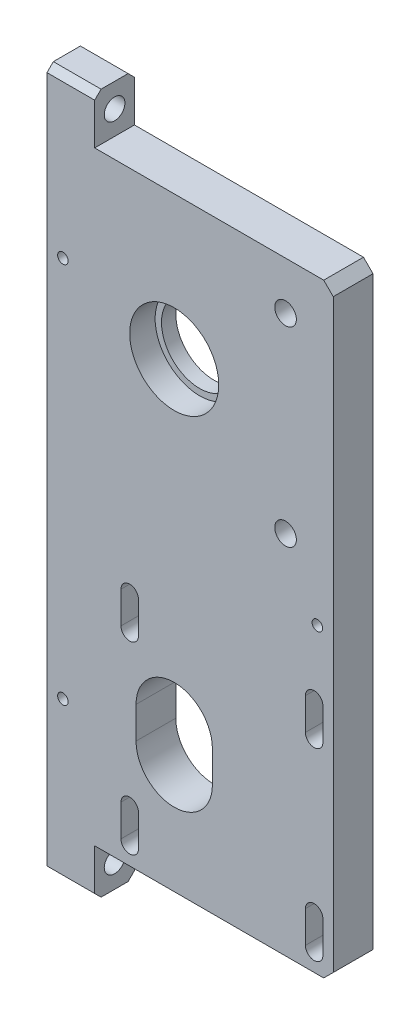
SolidWorks part; units mm, degrees
material "A6061"
ref_plane "前视基准面" through (0, 0, 0) normal (0, 0, 1) x (1, 0, 0)
ref_plane "上视基准面" through (0, 0, 0) normal (0, 1, 0) x (1, 0, 0)
ref_plane "右视基准面" through (0, 0, 0) normal (1, 0, 0) x (0, 0, -1)
sketch "草图1" plane through (0, 0, 0) normal (0, 0, 1) x (1, 0, 0)
  line L0 (0, 0) -> (-90, 0)
  line L1 (-90, 0) -> (-90, 220)
  line L2 (-90, 220) -> (0, 220)
  line L3 (0, 220) -> (0, 0)
  dimension "D1" = 220
  dimension "D4" = 90
extrude "凸台-拉伸1" add sketch "草图1" along normal blind 12.5
sketch "草图2" plane through (0, 0, 12.5) normal (0, 0, 1) x (1, 0, 0)
  line L0 (0, 220) -> (-90, 220) construction
  line L2 (-90, 220) -> (-90, 0) construction
  circle A0 centre (-50, 55) radius 12
  dimension "D1" = 165
  dimension "D2" = 40
  dimension "D3" = 24
extrude "切除-拉伸1" cut sketch "草图2" against normal through all
hole_wizard "打孔尺寸根据内六角圆柱头螺钉的类型1" positions "草图4" profile "草图3" counterbore size "M5" standard "Gb" end condition through all
sketch "草图4" plane through (0, 0, 12.5) normal (0, 0, 1) x (1, 0, 0)
  line L0 (-63.9914, 83.9914) -> (-6.0086, 26.0086) construction
  line L2 (-6.0086, 83.9914) -> (-63.9914, 26.0086) construction
  line L4 (-50, 55) -> (-35, 55) construction
  point P0 (-6.0086, 83.9914)
  point P2 (-6.0086, 26.0086)
  point P4 (-63.9914, 26.0086)
  point P6 (-63.9914, 83.9914)
  dimension "D1" = 45
  dimension "D2" = 90
  dimension "D3" = 15
  dimension "D4" = 82
  dimension "D5" = 82
sketch "草图3" plane through (-6.0086, 83.9914, 12.5) normal (1, 0, 0) x (0, -1, 0)
  line L0 (0, 0) -> (0, 12.5)
  line L1 (0, 12.5) -> (5, 12.5)
  line L3 (5, 12.5) -> (5, 6)
  line L4 (5, 6) -> (2.75, 6)
  line L5 (2.75, 6) -> (2.75, 0)
  line L7 (2.75, 0) -> (0, 0)
  line L11 (0, -6.35) -> (0, 107.95) construction
  dimension "通孔孔直径" = 10
  dimension "通孔孔深度" = 12.5
  dimension "柱形沉头孔直径" = 5.5
  dimension "柱形沉头孔深度" = 6
hole_wizard "M4 螺纹孔1" positions "草图7" profile "草图6" tap size "M4" standard "Gb" end condition through all
sketch "草图7" plane through (0, 0, 12.5) normal (0, 0, 1) x (1, 0, 0)
  line L0 (0, 220) -> (-90, 220) construction
  line L1 (-90, 220) -> (-90, 0) construction
  line L2 (-85, 50) -> (-85, 170) construction
  line L4 (-5, 110) -> (-85, 110) construction
  point P0 (-85, 170)
  point P3 (-85, 50)
  point P13 (-5, 110)
  dimension "D1" = 5
  dimension "D2" = 50
  dimension "D3" = 120
  dimension "D4" = 80
cosmetic thread "孔螺蚊线1" parameters "D2"=4
cosmetic thread "孔螺蚊线2" parameters "D2"=4
sketch "草图6" plane through (-85, 170, 12.5) normal (1, 0, 0) x (0, -1, 0)
  line L0 (0, 0) -> (0, 12.5)
  line L1 (0, 12.5) -> (1.65, 12.5)
  line L2 (1.65, 12.5) -> (1.65, 0)
  line L5 (1.65, 0) -> (0, 0)
  line L11 (0, -6.35) -> (0, 107.95) construction
  dimension "通孔螺纹孔钻头直径" = 3.3
  dimension "通孔螺纹孔钻头深度" = 12.5
cosmetic thread "孔螺蚊线5" parameters "D2"=4
sketch "草图12" plane through (0, 0, 0) normal (0, 0, -1) x (-1, 0, 0)
  line L0 (50, 50) -> (50, 60) construction
  line L1 (38, 50) -> (38, 60)
  line L2 (62, 50) -> (62, 60)
  line L3 (63.9914, 78.9914) -> (63.9914, 88.9914) construction
  line L4 (61.2414, 78.9914) -> (61.2414, 88.9914)
  line L5 (66.7414, 78.9914) -> (66.7414, 88.9914)
  line L6 (63.9914, 31.0086) -> (63.9914, 21.0086) construction
  line L7 (66.7414, 31.0086) -> (66.7414, 21.0086)
  line L8 (61.2414, 31.0086) -> (61.2414, 21.0086)
  line L9 (6.0086, 31.0086) -> (6.0086, 21.0086) construction
  line L10 (8.7586, 31.0086) -> (8.7586, 21.0086)
  line L11 (3.2586, 31.0086) -> (3.2586, 21.0086)
  line L12 (6.0086, 88.9914) -> (6.0086, 78.9914) construction
  line L13 (8.7586, 88.9914) -> (8.7586, 78.9914)
  line L14 (3.2586, 88.9914) -> (3.2586, 78.9914)
  arc A0 (38, 50) -> (62, 50) centre (50, 50) ccw
  arc A1 (62, 60) -> (38, 60) centre (50, 60) ccw
  arc A3 (61.2414, 78.9914) -> (66.7414, 78.9914) centre (63.9914, 78.9914) ccw
  arc A4 (66.7414, 88.9914) -> (61.2414, 88.9914) centre (63.9914, 88.9914) ccw
  arc A6 (66.7414, 31.0086) -> (61.2414, 31.0086) centre (63.9914, 31.0086) ccw
  arc A7 (61.2414, 21.0086) -> (66.7414, 21.0086) centre (63.9914, 21.0086) ccw
  arc A9 (8.7586, 31.0086) -> (3.2586, 31.0086) centre (6.0086, 31.0086) ccw
  arc A10 (3.2586, 21.0086) -> (8.7586, 21.0086) centre (6.0086, 21.0086) ccw
  arc A12 (8.7586, 88.9914) -> (3.2586, 88.9914) centre (6.0086, 88.9914) ccw
  arc A13 (3.2586, 78.9914) -> (8.7586, 78.9914) centre (6.0086, 78.9914) ccw
  circle A14 centre (50, 55) radius 12 construction
  circle A15 centre (6.0086, 83.9914) radius 2.75 construction
  circle A16 centre (63.9914, 83.9914) radius 2.75 construction
  circle A17 centre (63.9914, 26.0086) radius 2.75 construction
  circle A18 centre (6.0086, 26.0086) radius 2.75 construction
  point P2 (50, 55)
  point P7 (63.9914, 83.9914)
  point P17 (63.9914, 26.0086)
  point P27 (6.0086, 26.0086)
  point P37 (6.0086, 83.9914)
  dimension "D1" = 5.5
  dimension "D2" = 24
  dimension "D3" = 10
  dimension "D4" = 10
extrude "切除-拉伸5" cut sketch "草图12" against normal through all
sketch "草图13" plane through (0, 0, 0) normal (0, 0, -1) x (-1, 0, 0)
  line L0 (6.0086, 88.9914) -> (6.0086, 78.9914) construction
  line L1 (11.0086, 88.9914) -> (11.0086, 78.9914)
  line L2 (1.0086, 88.9914) -> (1.0086, 78.9914)
  line L3 (63.9914, 88.9914) -> (63.9914, 78.9914) construction
  line L4 (68.9914, 88.9914) -> (68.9914, 78.9914)
  line L5 (58.9914, 88.9914) -> (58.9914, 78.9914)
  line L6 (6.0086, 31.0086) -> (6.0086, 21.0086) construction
  line L7 (11.0086, 31.0086) -> (11.0086, 21.0086)
  line L8 (1.0086, 31.0086) -> (1.0086, 21.0086)
  line L9 (63.9914, 31.0086) -> (63.9914, 21.0086) construction
  line L10 (68.9914, 31.0086) -> (68.9914, 21.0086)
  line L11 (58.9914, 31.0086) -> (58.9914, 21.0086)
  arc A0 (11.0086, 88.9914) -> (1.0086, 88.9914) centre (6.0086, 88.9914) ccw
  arc A1 (1.0086, 78.9914) -> (11.0086, 78.9914) centre (6.0086, 78.9914) ccw
  arc A2 (68.9914, 88.9914) -> (58.9914, 88.9914) centre (63.9914, 88.9914) ccw
  arc A3 (58.9914, 78.9914) -> (68.9914, 78.9914) centre (63.9914, 78.9914) ccw
  arc A4 (11.0086, 31.0086) -> (1.0086, 31.0086) centre (6.0086, 31.0086) ccw
  arc A5 (1.0086, 21.0086) -> (11.0086, 21.0086) centre (6.0086, 21.0086) ccw
  arc A6 (68.9914, 31.0086) -> (58.9914, 31.0086) centre (63.9914, 31.0086) ccw
  arc A7 (58.9914, 21.0086) -> (68.9914, 21.0086) centre (63.9914, 21.0086) ccw
  point P4 (6.0086, 83.9914)
  point P9 (63.9914, 83.9914)
  point P18 (6.0086, 26.0086)
  point P27 (63.9914, 26.0086)
  dimension "D1" = 10
extrude "切除-拉伸6" cut sketch "草图13" against normal up to surface (6.5 mm away) up to face at (-2.1336, 83.9914, 6.5)
sketch "草图14" plane through (0, 0, 0) normal (0, 0, -1) x (-1, 0, 0)
  line L0 (0, 220) -> (90, 220) construction
  line L1 (90, 220) -> (90, 0) construction
  circle A0 centre (50, 160) radius 12
  dimension "D1" = 60
  dimension "D2" = 40
  dimension "D3" = 24
extrude "切除-拉伸7" cut sketch "草图14" against normal through all
sketch "草图15" plane through (0, 0, 12.5) normal (0, 0, 1) x (1, 0, 0)
  circle A0 centre (-50, 160) radius 14
  dimension "D1" = 28
extrude "切除-拉伸8" cut sketch "草图15" against normal blind 8
hole_wizard "M8 螺纹孔1" positions "草图17" profile "草图16" tap size "M8" standard "Gb" end condition through all
sketch "草图17" plane through (0, 0, 12.5) normal (0, 0, 1) x (1, 0, 0)
  line L0 (-50, 160) -> (-11.3553, 160) construction
  line L2 (-90, 220) -> (-90, 0) construction
  point P0 (-15, 130)
  point P2 (-15, 190)
  dimension "D1" = 60
  dimension "D2" = 75
sketch "草图16" plane through (-15, 130, 12.5) normal (1, 0, 0) x (0, -1, 0)
  line L0 (0, 0) -> (0, 12.5)
  line L1 (0, 12.5) -> (3.4, 12.5)
  line L2 (3.4, 12.5) -> (3.4, 0)
  line L5 (3.4, 0) -> (0, 0)
  line L11 (0, -6.35) -> (0, 107.95) construction
  dimension "通孔螺纹孔钻头直径" = 6.8
  dimension "通孔螺纹孔钻头深度" = 12.5
cosmetic thread "孔螺蚊线3" parameters "D2"=8
cosmetic thread "孔螺蚊线4" parameters "D2"=8
sketch "草图19" plane through (0, 0, 0) normal (1, 0, 0) x (0, 0, -1)
  line L0 (0, 0) -> (0, 220) construction
  line L1 (-12.5, 220) -> (0, 220)
  line L2 (-12.5, 220) -> (-12.5, 205)
  line L3 (-12.5, 205) -> (0, 205)
  line L4 (0, 220) -> (0, 205)
  line L6 (-12.5, 0) -> (0, 0)
  line L7 (-12.5, 0) -> (-12.5, 15)
  line L8 (-12.5, 15) -> (0, 15)
  line L9 (0, 0) -> (0, 15)
  dimension "D1" = 15
  dimension "D2" = 15
extrude "切除-拉伸10" cut sketch "草图19" against normal blind 75
chamfer "倒角1" distance 2 angle 45 4 edges at (-82.5, 220, 12.5) (-82.5, 220, 0) (-82.5, 0, 12.5) (-82.5, 0, 0)
chamfer "倒角2" distance 3 angle 45 2 edges at (0, 205, 6.25) (0, 15, 6.25)
sketch "草图20" plane through (-75, 0, 0) normal (1, 0, 0) x (0, 0, -1)
  line L0 (-2, 220) -> (-10.5, 220) construction
  line L1 (-20.5018, 110) -> (4.3418, 110) construction
  line L4 (-6.25, 220) -> (-6.25, 199.3114) construction
  line L5 (-12.5, 218) -> (-12.5, 205) construction
  line L6 (0, 205) -> (0, 218) construction
  circle A0 centre (-6.25, 212.5) radius 3.25
  circle A1 centre (-6.25, 7.5) radius 3.25
  dimension "D1" = 6.5
  dimension "D2" = 7.5
extrude "切除-拉伸11" cut sketch "草图20" against normal through all
